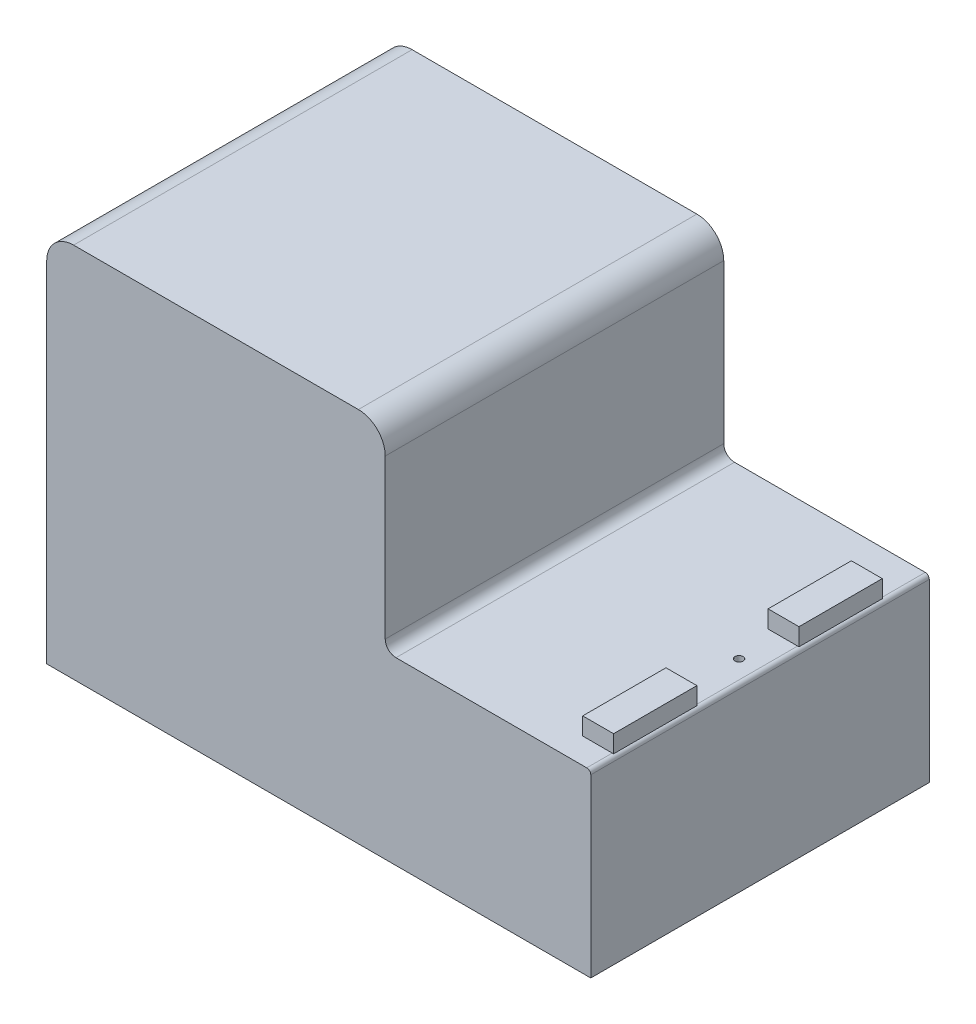
from build123d import *

# Parameters (mm, degrees)
EXTRUDE_1_DEPTH        = 63
FILLET_1_R             = 10
FILLET_2_R             = 1.5
SKETCH_2_R             = 1.5
CUT_EXTRUDE_1_DEPTH    = 10
SKETCH_3_W             = 11.5
SKETCH_3_H             = 31
EXTRUDE_2_DEPTH        = 6.5
FILLET_3_R             = 4
HOLE_WIZARD_M3_1_D     = 2.5
HOLE_WIZARD_M3_1_DEPTH = 11.5
HOLE_WIZARD_M3_1_TIP   = 0.751075774
SKETCH_6_W             = 45
SKETCH_6_H             = 70
SKETCH_6_H_2           = 75
CUT_EXTRUDE_2_DEPTH    = 10


with BuildPart() as part:
    # 草图1 → 凸台-拉伸1 (new, symmetric)
    with BuildSketch(Plane.XY):
        Polygon((0, 140), (0, 0), (202.5, 0), (202.5, 67), (126, 67), (126, 140), align=None)
    extrude(amount=EXTRUDE_1_DEPTH, both=True)

    # 圆角1
    fillet_1_edges = [part.edges().sort_by_distance(p)[0] for p in [
        (126, 140, 0),
        (0, 140, 0),
    ]]
    fillet(fillet_1_edges, radius=FILLET_1_R)

    # 圆角2
    fillet_2_edges = [part.edges().sort_by_distance(p)[0] for p in [
        (202.5, 67, 0),
    ]]
    fillet(fillet_2_edges, radius=FILLET_2_R)

    # 草图2 → 切除-拉伸1 (cut)
    with BuildSketch(Plane(origin=(0, 67, 0), x_dir=(1, 0, 0), z_dir=(0, 1, 0))):
        with Locations(Location((194.22, 0.5, 0), (0, 0, 180))):
            Circle(SKETCH_2_R)
    extrude(amount=-CUT_EXTRUDE_1_DEPTH, mode=Mode.SUBTRACT)

    # 草图3 → 凸台-拉伸2 (add)
    with BuildSketch(Plane(origin=(0, 67, 0), x_dir=(1, 0, 0), z_dir=(0, 1, 0))):
        with Locations((195.75, -38)):
            Rectangle(SKETCH_3_W, SKETCH_3_H)
        with Locations((195.75, 31)):
            Rectangle(SKETCH_3_W, SKETCH_3_H)
    extrude(amount=EXTRUDE_2_DEPTH)

    # 圆角3
    fillet_3_edges = [part.edges().sort_by_distance(p)[0] for p in [
        (126, 67, 0),
    ]]
    fillet(fillet_3_edges, radius=FILLET_3_R)

    # M3 螺纹孔1
    with Locations(Plane(origin=(0, 0, 0), x_dir=(-1, 0, 0), z_dir=(0, -1, 0))):
        with Locations((-16, -35), (-16, 35), (-186.5, -45), (-186.5, 45)):
            Hole(HOLE_WIZARD_M3_1_D / 2, depth=HOLE_WIZARD_M3_1_DEPTH)
            with Locations((0, 0, -(HOLE_WIZARD_M3_1_DEPTH + HOLE_WIZARD_M3_1_TIP / 2))):  # 118° drill point
                Cone(0, HOLE_WIZARD_M3_1_D / 2, HOLE_WIZARD_M3_1_TIP, mode=Mode.SUBTRACT)

    # 草图6 → 切除-拉伸2 (cut)
    with BuildSketch(Plane(origin=(0, 0, 0), x_dir=(-1, 0, 0), z_dir=(0, -1, 0))):
        with Locations((-76.5, 10)):
            Rectangle(SKETCH_6_W, SKETCH_6_H)
        with Locations((-142, -6.5)):
            Rectangle(SKETCH_6_W, SKETCH_6_H_2)
    extrude(amount=-CUT_EXTRUDE_2_DEPTH, mode=Mode.SUBTRACT)


solid = part.part
